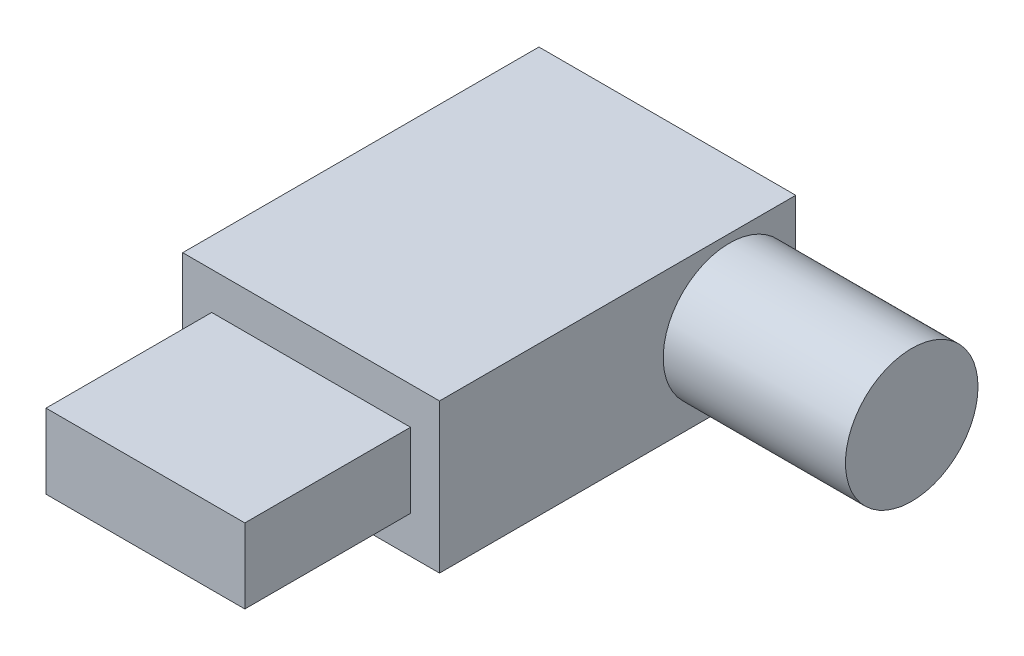
from build123d import *

# Parameters (mm, degrees)
SKETCH1_W           = 15.5
SKETCH1_H           = 9
BOSS_EXTRUDE1_DEPTH = 21.5
SKETCH2_R           = 4
BOSS_EXTRUDE2_DEPTH = 11
SKETCH3_W           = 12
SKETCH3_H           = 4.5
BOSS_EXTRUDE3_DEPTH = 10


with BuildPart() as part:
    # Sketch1 → Boss-Extrude1 (new body)
    with BuildSketch(Plane.XY):
        Rectangle(SKETCH1_W, SKETCH1_H)
    extrude(amount=-BOSS_EXTRUDE1_DEPTH)

    # Sketch2 → Boss-Extrude2 (add)
    with BuildSketch(Plane(origin=(7.75, 0, 0), x_dir=(0, 0, -1), z_dir=(1, 0, 0))):
        with Locations((17.5, 0)):
            Circle(SKETCH2_R)
    extrude(amount=BOSS_EXTRUDE2_DEPTH)

    # Sketch3 → Boss-Extrude3 (add)
    with BuildSketch(Plane.XY):
        Rectangle(SKETCH3_W, SKETCH3_H)
    extrude(amount=BOSS_EXTRUDE3_DEPTH)


solid = part.part
